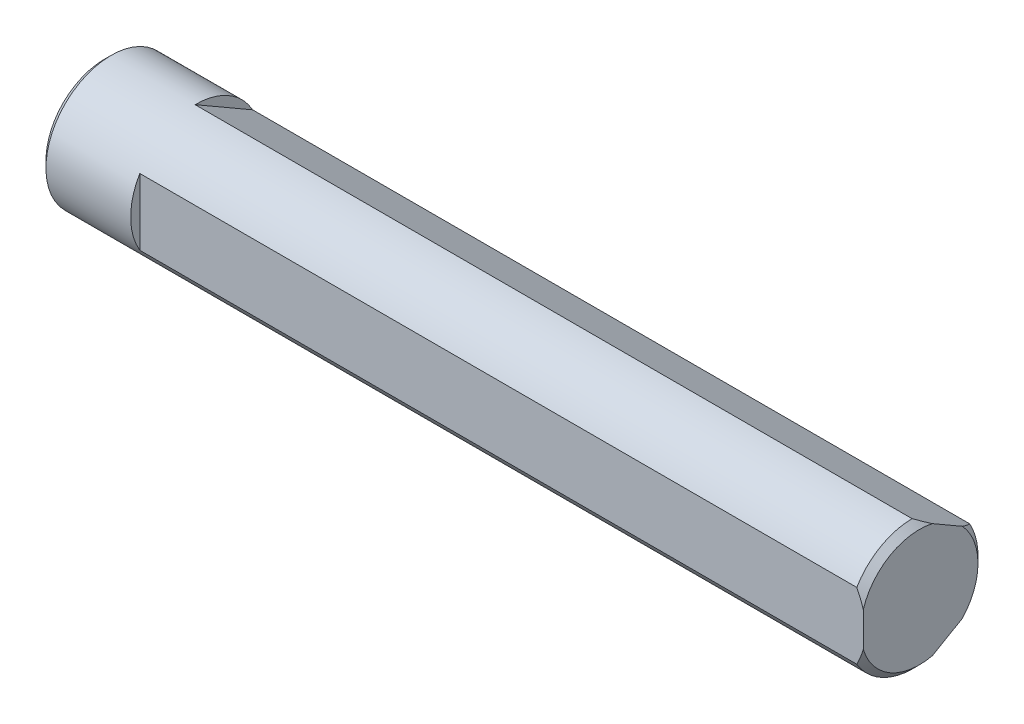
SolidWorks part; units mm, degrees
material "SUS304"
ref_plane "前视基准面" through (0, 0, 0) normal (0, 0, 1) x (1, 0, 0)
ref_plane "上视基准面" through (0, 0, 0) normal (0, 1, 0) x (1, 0, 0)
ref_plane "右视基准面" through (0, 0, 0) normal (1, 0, 0) x (0, 0, -1)
sketch "草图1" plane through (0, 0, 0) normal (1, 0, 0) x (0, 0, -1)
  circle A0 centre (0, 0) radius 5
  dimension "D1" = 10
extrude "凸台-拉伸1" add sketch "草图1" along normal blind 62.5
chamfer "倒角1" distance 0.5 angle 45 2 edges at (0, 0, -5) (62.5, 0, -5)
sketch "草图2" plane through (62.5, 0, 0) normal (1, 0, 0) x (0, 0, -1)
  line L1 (-8.7721, 6.3237) -> (-4.3, 6.3237)
  line L2 (-8.7721, 6.3237) -> (-8.7721, -6.5336)
  line L3 (-8.7721, -6.5336) -> (-4.3, -6.5336)
  line L4 (-4.3, 6.3237) -> (-4.3, -6.5336)
  circle A0 centre (0, 0) radius 5 construction
  dimension "D1" = 4.3
extrude "切除-拉伸1" cut sketch "草图2" against normal blind 55.5
pattern_circular "阵列(圆周)1" count 3 over 360 about axis through (0, 0, 0) along (1, 0, 0) of "切除-拉伸1"
hole_wizard "M4 螺纹孔1" positions "草图4" profile "草图3" tap size "M4" standard "GB"
sketch "草图4" plane through (0, 0, 0) normal (-1, 0, 0) x (0, 0, 1)
  point P0 (0, 0)
sketch "草图3" plane through (0, 0, 0) normal (0, 1, 0) x (0, 0, 1)
  line L0 (0, 0) -> (0, 16.4914)
  line L1 (0, 16.4914) -> (1.65, 15.5)
  line L2 (1.65, 15.5) -> (1.65, 0)
  line L5 (1.65, 0) -> (0, 0)
  line L10 (0, 16.4914) -> (-1.65, 15.5) construction
  line L11 (0, -6.35) -> (0, 107.95) construction
  dimension "螺纹孔钻头直径" = 3.3
  dimension "螺纹孔钻头深度" = 15.5
  dimension "导头角度" = 118
cosmetic thread "孔螺蚊线1" parameters "D1"=12, "D2"=4
